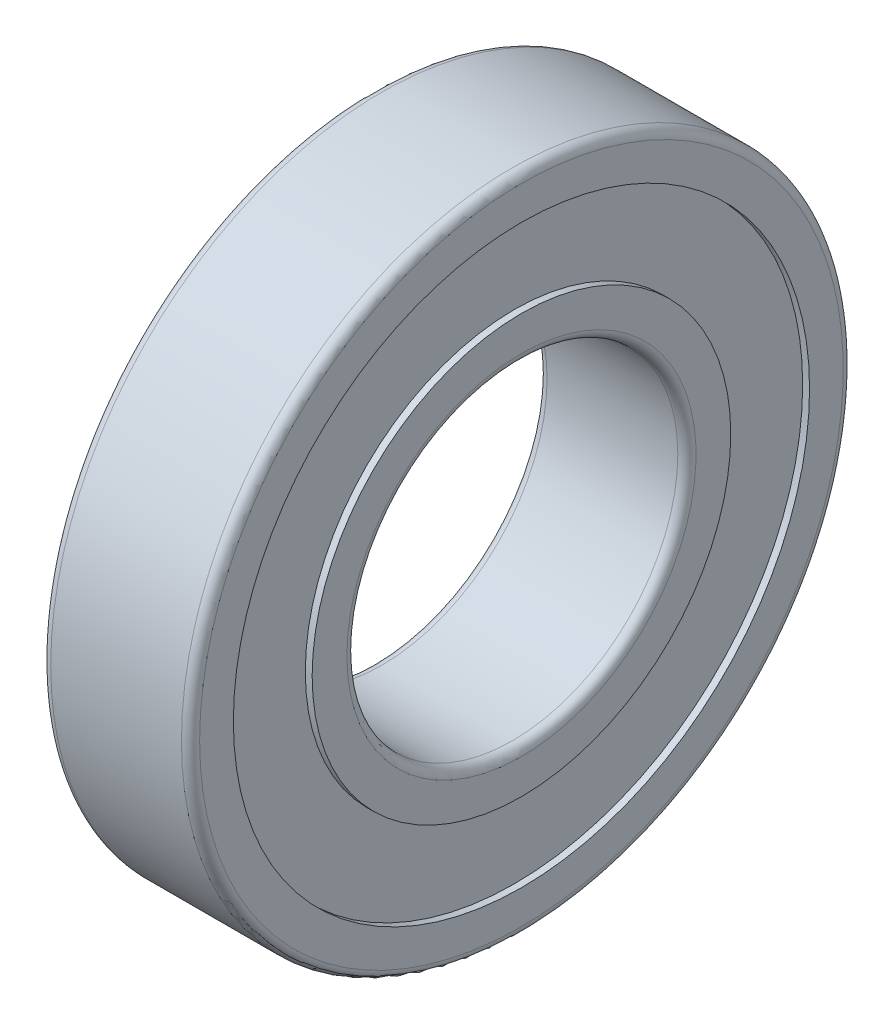
from build123d import *

# Parameters (mm, degrees)
FILLET1_R = 1.1
FILLET2_R = 1.1


with BuildPart() as part:
    # Sketch1 → Revolve1 (revolve)
    with BuildSketch(Plane.XY, mode=Mode.PRIVATE) as revolve1_sk:
        Polygon((0, 20), (18, 20), (18, 25.3), (17.17, 25.3), (17.17, 34.825), (18, 34.825), (18, 40), (0, 40), (0, 34.825), (0.83, 34.825), (0.83, 25.3), (0, 25.3), align=None)
    revolve(revolve1_sk.sketch.rotate(Axis((0, 0, 0), (1, 0, 0)), 90), axis=Axis((0, 0, 0), (1, 0, 0)))

    # Fillet1
    fillet1_edges = [part.edges().sort_by_distance(p)[0] for p in [
        (0, 0, -40),
        (18, 0, -40),
    ]]
    fillet(fillet1_edges, radius=FILLET1_R)

    # Fillet2
    fillet2_edges = [part.edges().sort_by_distance(p)[0] for p in [
        (18, 0, -20),
        (0, 0, -20),
    ]]
    fillet(fillet2_edges, radius=FILLET2_R)


solid = part.part
